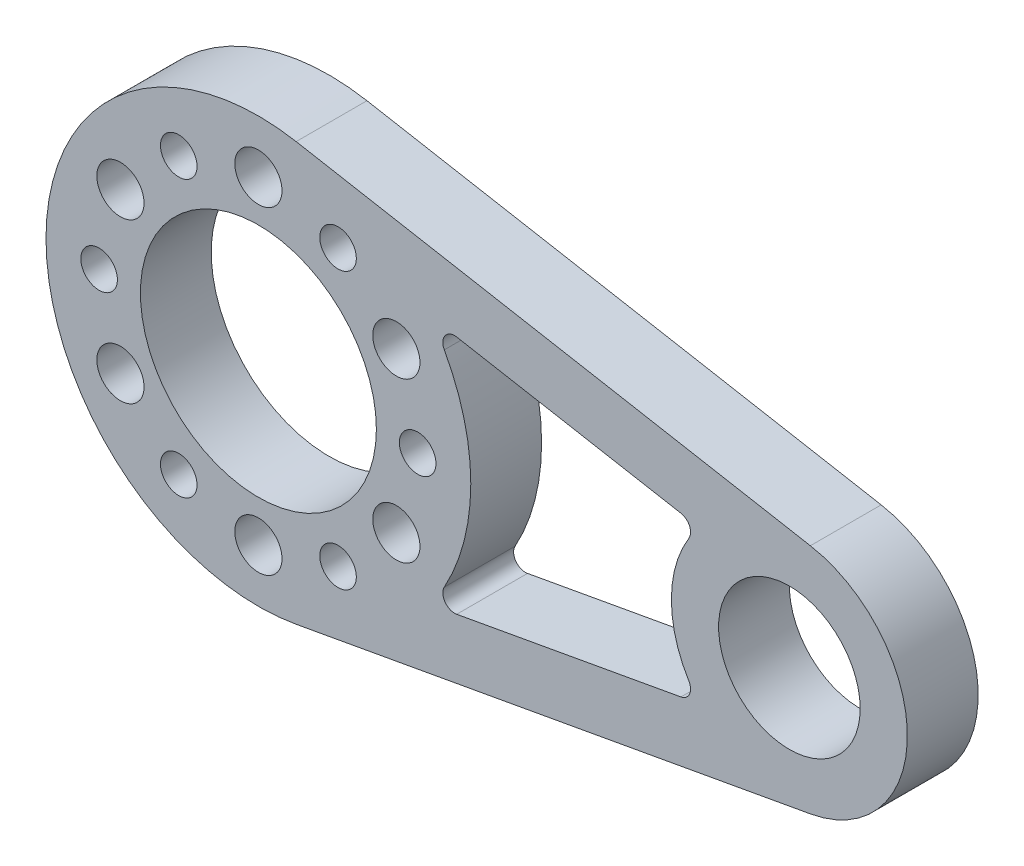
SolidWorks part; units mm, degrees
material "Thornel Mat VMA"
ref_plane "前视基准面" through (0, 0, 0) normal (0, 0, 1) x (1, 0, 0)
ref_plane "上视基准面" through (0, 0, 0) normal (0, 1, 0) x (1, 0, 0)
ref_plane "右视基准面" through (0, 0, 0) normal (1, 0, 0) x (0, 0, -1)
other "Configuration Table"
sketch "草图1" plane through (0, 0, 0) normal (0, 0, 1) x (1, 0, 0)
  line L0 (0, 0) -> (45, 0) construction
  line L1 (0, 0) -> (13.5, 0) construction
  line L2 (3.2, 17.7133) -> (46.7778, 9.8407)
  line L3 (3.2, -17.7133) -> (46.7778, -9.8407)
  line L4 (0, 13.5) -> (0, 0) construction
  circle A0 centre (45, 0) radius 6
  circle A1 centre (0, 0) radius 13.5 construction
  circle A2 centre (13.5, 0) radius 1.55
  circle A3 centre (6.75, -11.6913) radius 1.55
  circle A4 centre (-6.75, -11.6913) radius 1.55
  circle A5 centre (-13.5, 0) radius 1.55
  circle A6 centre (-6.75, 11.6913) radius 1.55
  circle A7 centre (6.75, 11.6913) radius 1.55
  circle A8 centre (0, 0) radius 18
  circle A9 centre (45, 0) radius 10
  circle A10 centre (0, 0) radius 10
  circle A11 centre (0, 13.5) radius 2
  circle A12 centre (11.6913, 6.75) radius 2
  circle A13 centre (11.6913, -6.75) radius 2
  circle A14 centre (0, -13.5) radius 2
  circle A15 centre (-11.6913, -6.75) radius 2
  circle A16 centre (-11.6913, 6.75) radius 2
  point P19 (0, 0)
  point P39 (0, 0)
  dimension "D1" = 12
  dimension "D3" = 27
  dimension "D6" = 3.1
  dimension "D7" = 20
  dimension "D8" = 36
  dimension "D9" = 20
  dimension "D11" = 4
  dimension "D2" = 45
  dimension "D5" = 0
  dimension "D4" = 6
  dimension "D10" = 6
extrude "凸台-拉伸1" add sketch "草图1" along normal blind 6 contours A8 A2 A3 A4 A5 A6 A7 | A9 L2 A8 L3 | A9 A0
sketch "草图2" plane through (0, 0, 6) normal (0, 0, 1) x (1, 0, 0)
  line L0 (0, 0) -> (45, 0)
sketch "草图3" plane through (0, 0, 6) normal (0, 0, 1) x (1, 0, 0)
  line L0 (14.5627, 10.5796) -> (37.3666, 6.46)
  line L1 (3.2, 17.7133) -> (46.7778, 9.8407) construction
  line L2 (45, 0) -> (-0.4013, 0) construction
  line L3 (14.5627, -10.5796) -> (37.3666, -6.46)
  circle A0 centre (0, 0) radius 18
  arc A1 (3.2, 17.7133) -> (3.2, -17.7133) centre (0, 0) ccw construction
  circle A2 centre (45, 0) radius 10
  dimension "D1" = 20
  dimension "D2" = 5
extrude "切除-拉伸1" cut sketch "草图3" against normal through all contours L2 A2 L0 A0 | A2 L2 A0 L3
fillet "圆角1" radius 1 4 edges at (14.5627, -10.5796, 3) (37.3666, -6.46, 3) (37.3666, 6.46, 3) (14.5627, 10.5796, 3)
